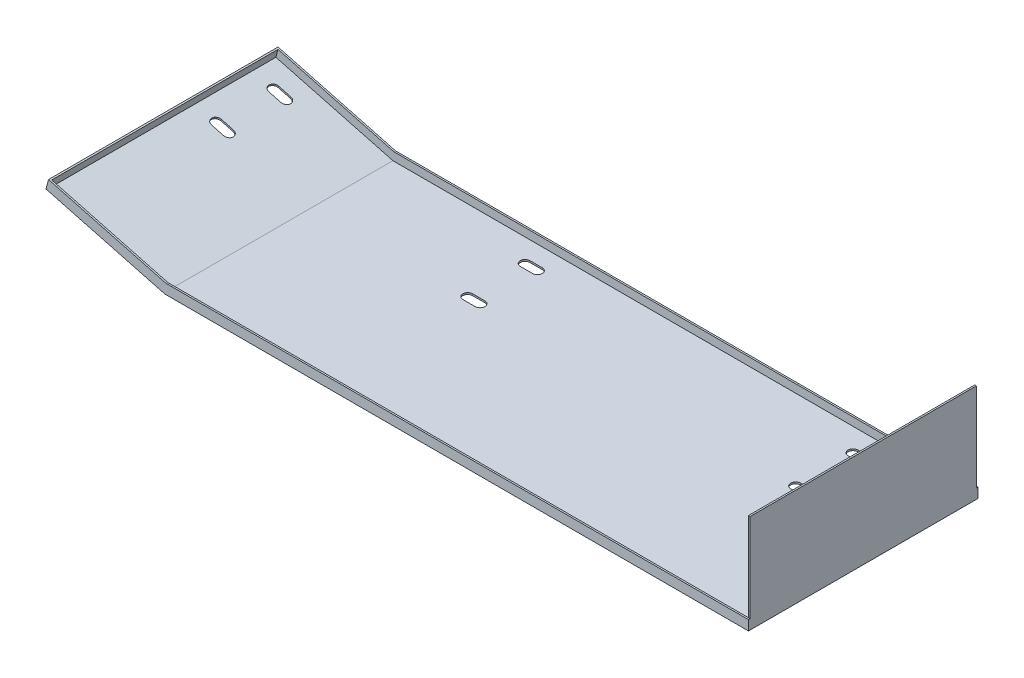
from build123d import *

# Parameters (mm, degrees)
EXTRUDE_THIN1_DEPTH  = 276
EXTRUDE_THIN2_DEPTH  = 2
EXTRUDE_THIN3_DEPTH  = 2
CUT_EXTRUDE1_DEPTH   = 2
CUT_EXTRUDE2_DEPTH   = 2
SKETCH7_W            = 2
SKETCH7_H            = 276
BOSS_EXTRUDE1_DEPTH  = 10
LPATTERN1_COUNT      = 2
LPATTERN1_PITCH      = 70
LPATTERN2_COUNT      = 2
LPATTERN2_PITCH      = 70
LPATTERN2_COUNT_DIR2 = 2
LPATTERN2_PITCH_DIR2 = 400


with BuildPart() as part:
    # Sketch1 → Extrude-Thin1 (new body)
    with BuildSketch(Plane.XY):
        Polygon((-856.990015303, 38.44340597), (-712, 0), (0, 0), (0, 120), (-2, 120), (-2, 2), (-711.739357917, 2), (-856.477436556, 40.376606174), align=None)
    extrude(amount=EXTRUDE_THIN1_DEPTH)

    # Sketch2 → Extrude-Thin2 (add)
    with BuildSketch(Plane.XY.offset(276)):
        Polygon((0, 0), (-712, 0), (-856.990015303, 38.44340597), (-853.914542825, 50.042607194), (-710.436147504, 12), (0, 12), align=None)
    extrude(amount=EXTRUDE_THIN2_DEPTH)

    # Sketch4 → Extrude-Thin3 (add)
    with BuildSketch(Plane(origin=(0, 0, 0), x_dir=(-1, 0, 0), z_dir=(0, 0, -1))):
        Polygon((0, 0), (712, 0), (856.990015303, 38.44340597), (853.914542825, 50.042607194), (710.436147504, 12), (0, 12), align=None)
    extrude(amount=EXTRUDE_THIN3_DEPTH)

    # Sketch5 → Cut-Extrude1 (cut)
    with BuildSketch(Plane.XZ):
        with BuildLine():
            Line((-122.5, 34), (-107.5, 34))
            ThreePointArc((-107.5, 34), (-101.5, 28), (-107.5, 22))
            Line((-107.5, 22), (-122.5, 22))
            ThreePointArc((-122.5, 22), (-128.5, 28), (-122.5, 34))
        make_face()
    cut_extrude1 = extrude(amount=-CUT_EXTRUDE1_DEPTH, mode=Mode.SUBTRACT)

    # Sketch6 → Cut-Extrude2 (cut)
    with BuildSketch(Plane(origin=(-46.76718086, -176.383285962, 0), x_dir=(0.9666001020169073, -0.2562893731329973, 0), z_dir=(-0.2562893731329973, -0.9666001020169073, 0))):
        with BuildLine():
            Line((-809.719272636, 34), (-794.719272636, 34))
            ThreePointArc((-794.719272636, 34), (-788.719272636, 28), (-794.719272636, 22))
            Line((-794.719272636, 22), (-809.719272636, 22))
            ThreePointArc((-809.719272636, 22), (-815.719272636, 28), (-809.719272636, 34))
        make_face()
    cut_extrude2 = extrude(amount=-CUT_EXTRUDE2_DEPTH, mode=Mode.SUBTRACT)

    # Sketch7 → Boss-Extrude1 (add)
    with BuildSketch(Plane(origin=(-46.254602114, -174.450085758, 0), x_dir=(0.9666001020169073, -0.25628937313299727, 0), z_dir=(0.25628937313299727, 0.9666001020169073, 0))):
        with Locations((-837.219272636, -138)):
            Rectangle(SKETCH7_W, SKETCH7_H)
    extrude(amount=BOSS_EXTRUDE1_DEPTH)

    # LPattern1: Cut-Extrude2 ×2
    with Locations(*[(0, 0, i * LPATTERN1_PITCH) for i in range(1, LPATTERN1_COUNT)]):
        add(cut_extrude2, mode=Mode.SUBTRACT)

    # LPattern2: Cut-Extrude1 2 × 2
    with Locations(*[(-j * LPATTERN2_PITCH_DIR2, 0, i * LPATTERN2_PITCH) for i in range(LPATTERN2_COUNT) for j in range(LPATTERN2_COUNT_DIR2) if (i, j) != (0, 0)]):
        add(cut_extrude1, mode=Mode.SUBTRACT)


solid = part.part
